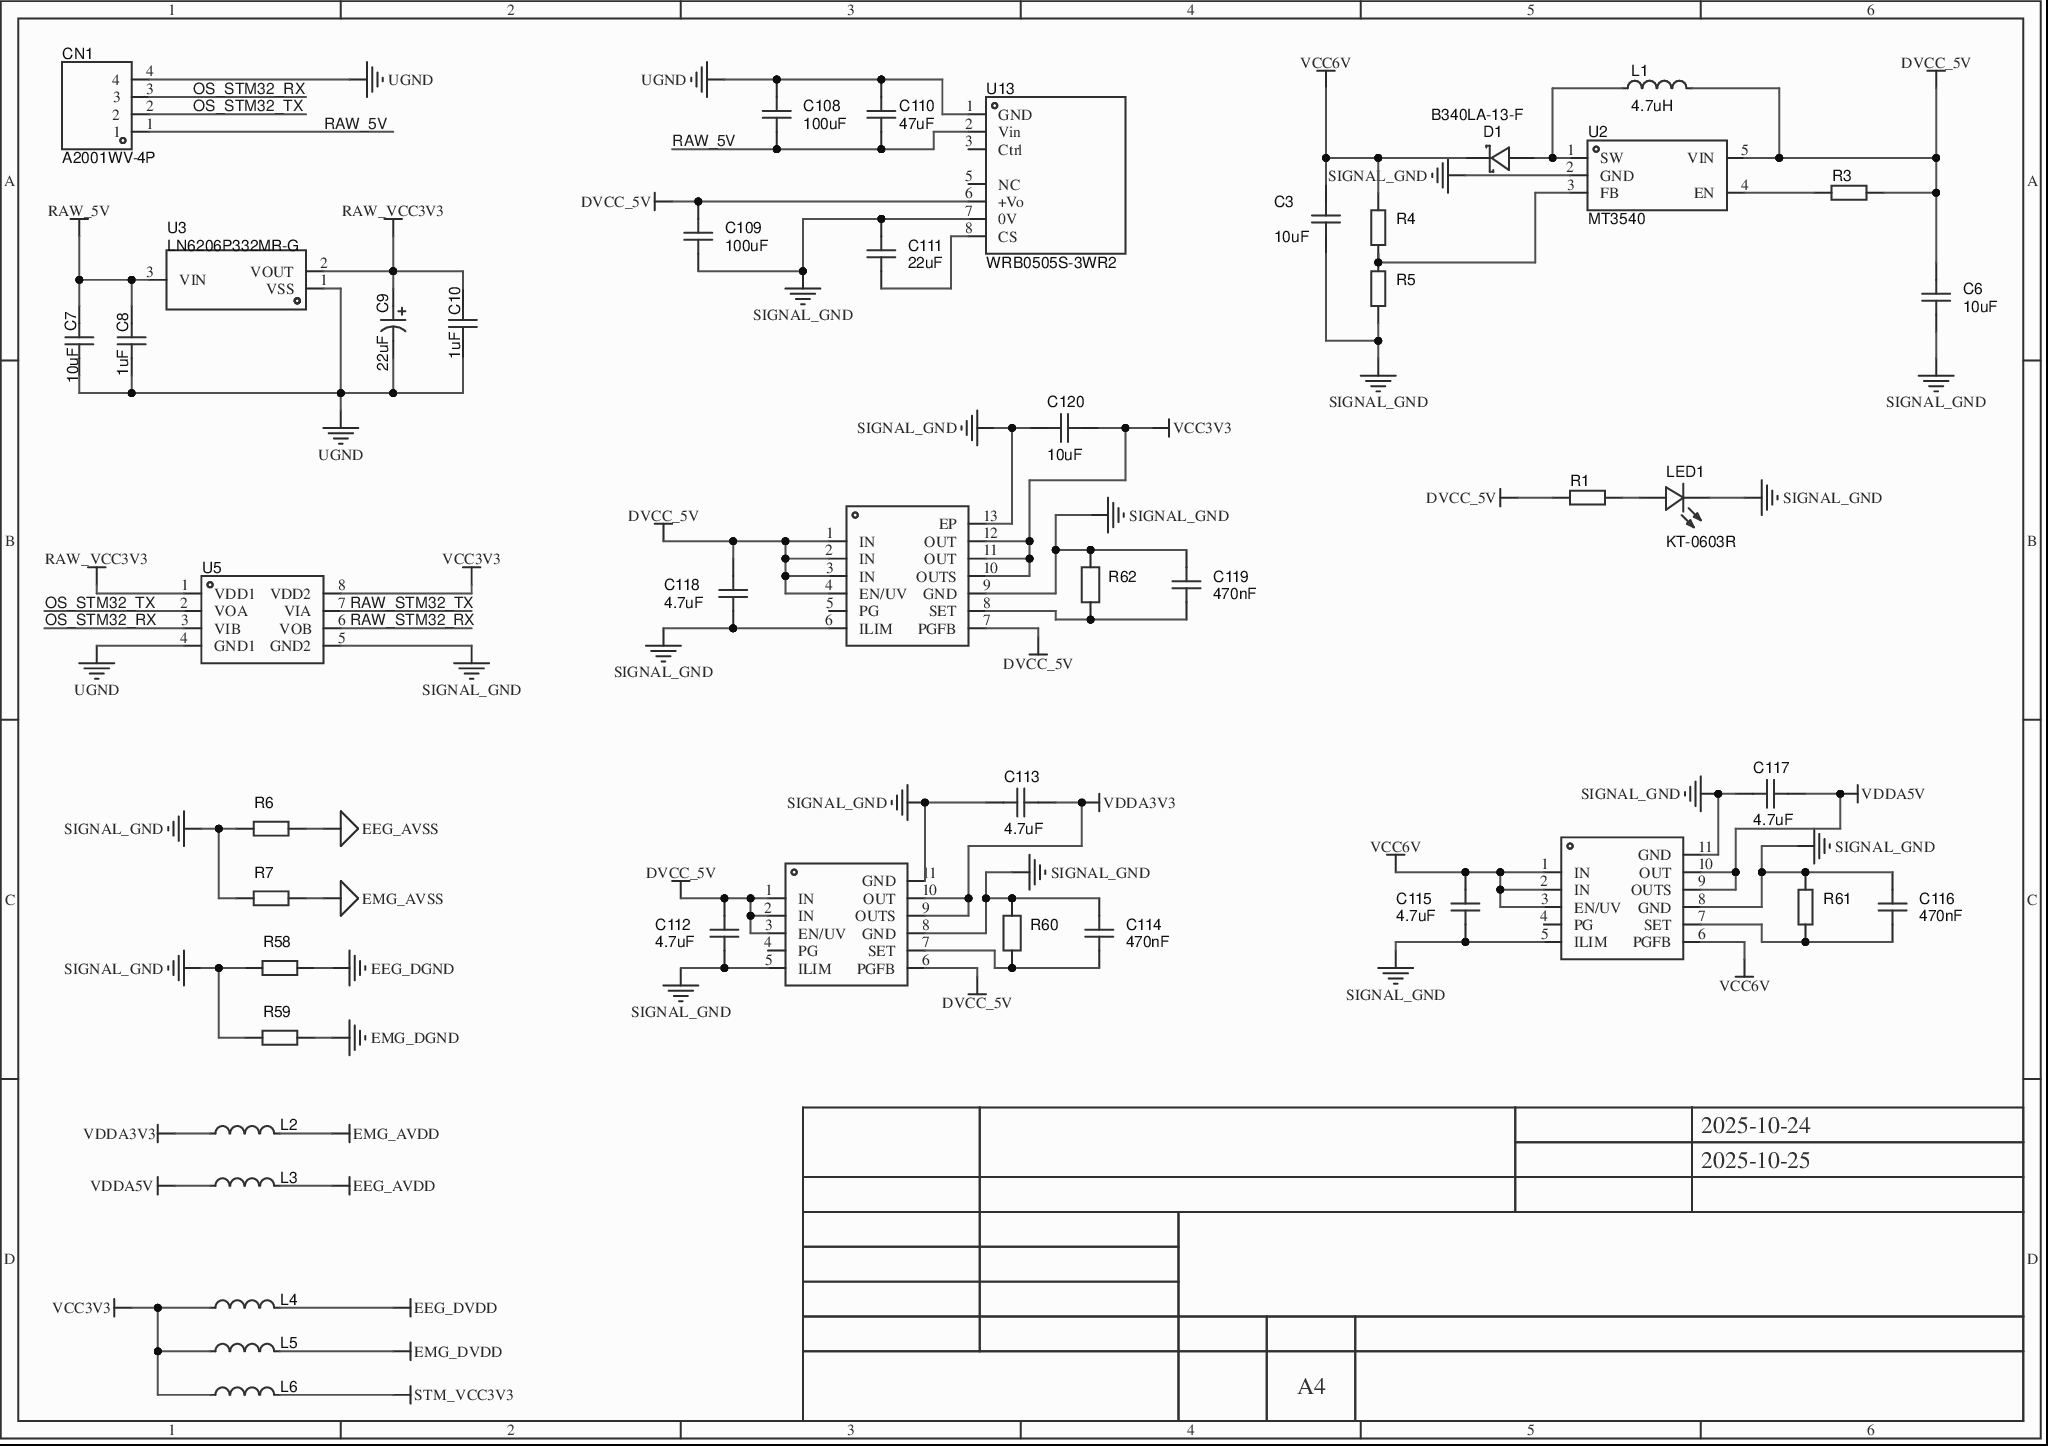
[diagram p0: MISC86293-47.schdoc]
# Altium project MISC86293-17.PrjPCB (part 1 of 3)
8 sheets, 211 parts. Net scope: global (net labels, ports and power ports of the same name join across sheets).
Board file: MISC86293.PcbDoc
Sheets:
  MISC86293-47.schdoc
  MISC86293-6.schdoc
  MISC86293-8.schdoc
  MISC86293-4.schdoc
  MISC86293-12.schdoc
  MISC86293-21.schdoc
  MISC86293-14.schdoc
  MISC86293-10.schdoc

## Sheet MISC86293-47.schdoc
size 297 x 209 mm; Version: V1.0; @Project Name: MISC86293; @Page Count: 8; @Update Date: 2025-10-25; @Create Date: 2025-10-24; @Schematic Name: MISC86293; @Page No: 1; @Create Time: 20:02:05; @Update Time: 11:40:48; @Board Name: MISC86293

### Parts
C3  10uF  [C0603]
C6  10uF  [C0603]
C7  10uF  [C0603]
C8  1uF  [C0402]
C9  22uF  [CAP-SMD_L3.2-W1.6]
C10  1uF  [C0402]
C108  100uF  [C1206]
C109  100uF  [C1206]
C110  47uF  [C1206]
C111  22uF  [C1206]
C112  4.7uF  [C0603]
C113  4.7uF  [C0603]
C114  470nF  [C0603]
C115  4.7uF  [C0603]
C116  470nF  [C0603]
C117  4.7uF  [C0603]
C118  4.7uF  [C0603]
C119  470nF  [C0603]
C120  10uF  [C0603]
CN1  A2001WV-4P  [CONN-TH_A2001WV-4P]
D1  B340LA-13-F  [SMA_L4.3-W2.6-LS5.2-RD]
L1  4.7uH  [IND-SMD_L4.0-W4.0_FNR40XXS]
L2  BLM15PD121SN1D  [L0402]  (value not drawn)
L3  BLM15PD121SN1D  [L0402]  (value not drawn)
L4  BLM15PD121SN1D  [L0402]  (value not drawn)
L5  BLM15PD121SN1D  [L0402]  (value not drawn)
L6  BLM15PD121SN1D  [L0402]  (value not drawn)
LED1  KT-0603R  [LED0603-RD]
R1  (no value)  [R0603]
R3  (no value)  [R0402]
R4  (no value)  [R0402]
R5  (no value)  [R0402]
R6  (no value)  [R0402]
R7  (no value)  [R0402]
R58  (no value)  [R0402]
R59  (no value)  [R0402]
R60  (no value)  [R0603]
R61  (no value)  [R0603]
R62  (no value)  [R0603]
U2  MT3540  [SOT-23-5_L3.0-W1.7-P0.95-LS2.8-BR]
U3  LN6206P332MR-G  [SOT-23-3_L2.9-W1.3-P1.90-LS2.4-BR]
U5  (no value)  [SOIC-8_L4.9-W3.9-P1.27-LS6.0-BL]
U13  WRB0505S-3WR2  [PWRM-TH_WRA0512S-3WR2]
U14  LT3045EMSE#TRPBF  [MSOP-12_L4.0-W3.0-P0.65-LS4.9-BL-EP]  (value not drawn)
U15  LT3042EMSE#TRPBF  [MSOP-10_L3.0-W3.0-P0.50-LS5.0-BL-EP]  (value not drawn)
U16  LT3042EMSE#TRPBF  [MSOP-10_L3.0-W3.0-P0.50-LS5.0-BL-EP]  (value not drawn)

### Nets
DVCC_5V: C6.2 C109.1 C112.2 C118.2 L1.2 R1.1 R3.2 U2.5(VIN) U13.6(+Vo) U14.1(IN) U14.2(IN) U14.3(IN) U14.4(EN/UV) U14.7(PGFB) U15.1(IN) U15.2(IN) U15.3(EN/UV) U15.6(PGFB)
EEG_AVDD: L3.2  [project net EEG_AVDD1]
EEG_AVSS: R6.1  [project net EEG_AVSS1]
EEG_DGND: R58.1  [project net EEG_DGND_1]
EEG_DVDD: L4.2  [project net EEG_DVDD_1]
EMG_AVDD: L2.2  [project net EMG_AVDD1]
EMG_AVSS: R7.1  [project net EMG_AVSS1]
EMG_DGND: R59.1  [project net EMG_DGND_1]
EMG_DVDD: L5.2  [project net EMG_DVDD_1]
RAW_5V: C7.2 C8.2 C108.1 C110.1 CN1.1 U3.3(VIN) U13.2(Vin)
RAW_VCC3V3: C9.1 C10.2 U3.2(VOUT) U5.1(VDD1)
SIGNAL_GND: C3.1 C6.1 C109.2 C111.2 C112.1 C113.2 C114.1 C115.1 C116.1 C117.2 C118.1 C119.1 C120.1 LED1.1(K) R5.1 R6.2 R7.2 R58.2 R59.2 R60.1 R61.2 R62.1 U2.2(GND) U5.5(GND2) U13.7(0V) U14.6(ILIM) U14.9(GND) U14.13(EP) U15.5(ILIM) U15.8(GND) U15.11(GND) U16.5(ILIM) U16.8(GND) U16.11(GND)
STM_VCC3V3: L6.2
UGND: C7.1 C8.1 C9.2 C10.1 C108.2 C110.2 CN1.4 U3.1(VSS) U5.4(GND1) U13.1(GND)
VCC3V3: C120.2 L4.1 L5.1 L6.1 U5.8(VDD2) U14.10(OUTS) U14.11(OUT) U14.12(OUT)
VCC6V: C3.2 C115.2 D1.1(K) R4.2 U16.1(IN) U16.2(IN) U16.3(EN/UV) U16.6(PGFB)
VDDA3V3: C113.1 L2.1 U15.9(OUTS) U15.10(OUT)
VDDA5V: C117.1 L3.1 U16.9(OUTS) U16.10(OUT)
OS_STM32_RX: CN1.3 U5.3(VIB)
OS_STM32_TX: CN1.2 U5.2(VOA)
RAW_STM32_RX: U5.6(VOB)
RAW_STM32_TX: U5.7(VIA)
NetC111_1: C111.1 U13.8(CS)
NetC114_2: C114.2 R60.2 U15.7(SET)
NetC116_2: C116.2 R61.1 U16.7(SET)
NetC119_2: C119.2 R62.2 U14.8(SET)
NetD1_2: D1.2(A) L1.1 U2.1(SW)
NetLED1_2: LED1.2(A) R1.2
NetR3_1: R3.1 U2.4(EN)
NetR4_1: R4.1 R5.2 U2.3(FB)

Not connected (* = marked no-connect by the designer): U13 3(Ctrl)* 5(NC)*; U14 5(PG)*; U15 4(PG)*; U16 4(PG)*

### Notes on the sheet
- 1
- 2
- 3
- 4
- 5
- 6
- A
- B
- C
- 2025-10-24
- 2025-10-25
- D
- A4

### Library data of the parts
C3 C6 = CL10A106MA8NRNC: AddInBom: yes; ModelId: ac125912035d415993ca9572d50418b1; ModelName: C0603_L1.6-W0.8-H0.8; ModelTransform: 62.992,31.496,0,0,0,0,0,0,0; Voltage Rated: 25V; Temperature Coefficient: X5R; Symbol: CL10A106MA8NRNC; Device: CL10A106MA8NRNC; Supplier: LCSC; Manufacturer Part: CL10A106MA8NRNC; Value: 10uF; Supplier Part: C96446; Supplier Footprint: 0603; Datasheet: https://atta.szlcsc.com/upload/public/pdf/source/20160218/1457707763339.pdf; ConvertToPcb: yes; FootprintName: C0603
C7 = CL10A106KP8NNNC: AddInBom: yes; ModelId: ac125912035d415993ca9572d50418b1; ModelName: C0603_L1.6-W0.8-H0.8; ModelTransform: 62.992,31.496,0,0,0,0,0,0,0; Voltage Rated: 10V; Temperature Coefficient: X5R; Symbol: CL10A106KP8NNNC; Device: CL10A106KP8NNNC; Supplier: LCSC; Manufacturer Part: CL10A106KP8NNNC; Value: 10uF; Supplier Part: C19702; Supplier Footprint: 0603; Datasheet: https://atta.szlcsc.com/upload/public/pdf/source/20160218/1457707763339.pdf; ConvertToPcb: yes; FootprintName: C0603
C8 C10 = CL05A105KA5NQNC: AddInBom: yes; ModelId: 36a51122f27c49738f86b3bfa98863e0; ModelName: C0402_L1.0-W0.5-H0.5; ModelTransform: 39.37,19.685,0,0,0,0,0,0,0; Voltage Rated: 25V; Temperature Coefficient: X5R; Symbol: CL05A105KA5NQNC; Device: CL05A105KA5NQNC; SupplierPart: C52923; ManufacturerPart: CL05A105KA5NQNC; Supplier Footprint: 0402; JLCPCB Part Class: Basic Part; Datasheet: https://atta.szlcsc.com/upload/public/pdf/source/20160218/1457707763339.pdf; Supplier: LCSC; ConvertToPcb: yes; FootprintName: C0402; Value: 1uF
C9 = CA45-A-16V-22uF-K: AddInBom: yes; ModelId: 16e6b9a38ba84019a70b57c5f1368526; ModelTransform: 125.984,62.992,0,0,0,0,0,0,0; Rated Voltage: 16V; Device: CA45-A-16V-22uF-K; Symbol: CA45-A-16V-22UF-K; SupplierPart: C782264; ManufacturerPart: CA45-A-16V-22uF-K; Supplier Footprint: CASE-A-3216; Datasheet: https://atta.szlcsc.com/upload/public/pdf/source/20200909/C782264_D6D9C4EF3B25E81633C26A9294FBB820.pdf; Supplier: LCSC; ConvertToPcb: yes; FootprintName: CAP-SMD_L3.2-W1.6; ModelName: CAP-SMD_L3.2-W1.6; Value: 22uF
C108 C109 = GRM31CR61A107MEA8L: AddInBom: yes; ModelId: e4be705b945545a48e666415e3682bd8; ModelName: C1206_L3.2-W1.6-H1.3; ModelTransform: 125.984,62.992,0,0,0,0,0,0,0; Voltage Rating: 10V; Temperature Coefficient: X5R; Symbol: GRM31CR61A107MEA8L; Device: GRM31CR61A107MEA8L; Value: 100uF; SupplierPart: C883598; ManufacturerPart: GRM31CR61A107MEA8L; Supplier Footprint: 1206; JLCPCB Part Class: Extended Part; Datasheet: https://item.szlcsc.com/datasheet/GRM31CR61A107MEA8L/948963.html; Supplier: LCSC; ConvertToPcb: yes; FootprintName: C1206
C110 = GRM31CR61A476ME15L: AddInBom: yes; ModelId: e4be705b945545a48e666415e3682bd8; ModelName: C1206_L3.2-W1.6-H1.3; ModelTransform: 125.984,62.992,0,0,0,0,0,0,0; Voltage Rating: 10V; Temperature Coefficient: X5R; Symbol: GRM31CR61A476ME15L; Device: GRM31CR61A476ME15L; Value: 47uF; SupplierPart: C94034; ManufacturerPart: GRM31CR61A476ME15L; Supplier Footprint: 1206; JLCPCB Part Class: Extended Part; Datasheet: https://item.szlcsc.com/datasheet/GRM31CR61A476ME15L/95232.html; Supplier: LCSC; ConvertToPcb: yes; FootprintName: C1206
C111 = GRM31CR71A226KE15L: AddInBom: yes; ModelId: e4be705b945545a48e666415e3682bd8; ModelName: C1206_L3.2-W1.6-H1.3; ModelTransform: 125.984,62.992,0,0,0,0,0,0,0; Voltage Rating: 10V; Temperature Coefficient: X7R; Symbol: GRM31CR71A226KE15L; Device: GRM31CR71A226KE15L; Value: 22uF; SupplierPart: C91604; ManufacturerPart: GRM31CR71A226KE15L; Supplier Footprint: 1206; JLCPCB Part Class: Extended Part; Datasheet: https://item.szlcsc.com/datasheet/GRM31CR71A226KE15L/92793.html; Supplier: LCSC; ConvertToPcb: yes; FootprintName: C1206
C112 C113 C115 C117 C118 = GRM188Z71C475KE21D: AddInBom: yes; ModelId: ac125912035d415993ca9572d50418b1; ModelName: C0603_L1.6-W0.8-H0.8; ModelTransform: 62.992,31.496,0,0,0,0,0,0,0; Voltage Rating: 16V; Temperature Coefficient: X7R; Symbol: GRM188Z71C475KE21D; Device: GRM188Z71C475KE21D; Value: 4.7uF; SupplierPart: C389010; ManufacturerPart: GRM188Z71C475KE21D; Supplier Footprint: 0603; JLCPCB Part Class: Extended Part; Datasheet: https://item.szlcsc.com/datasheet/GRM188Z71C475KE21D/364359.html; Supplier: LCSC; ConvertToPcb: yes; FootprintName: C0603
C114 C116 C119 = GRM188R71A474KA61D: AddInBom: yes; ModelId: ac125912035d415993ca9572d50418b1; ModelName: C0603_L1.6-W0.8-H0.8; ModelTransform: 62.992,31.496,0,0,0,0,0,0,0; Voltage Rating: 10V; Temperature Coefficient: X7R; Symbol: GRM188R71A474KA61D; Device: GRM188R71A474KA61D; Value: 470nF; SupplierPart: C435402; ManufacturerPart: GRM188R71A474KA61D; Supplier Footprint: 0603; JLCPCB Part Class: Extended Part; Datasheet: https://item.szlcsc.com/datasheet/GRM188R71A474KA61D/432740.html; Supplier: LCSC; ConvertToPcb: yes; FootprintName: C0603
C120 = GRM188Z71A106KA73D: AddInBom: yes; ModelId: ac125912035d415993ca9572d50418b1; ModelName: C0603_L1.6-W0.8-H0.8; ModelTransform: 62.992,31.496,0,0,0,0,0,0,0; Voltage Rated: 10V; Temperature Coefficient: X7R; Symbol: GRM188Z71A106KA73D; Device: GRM188Z71A106KA73D; SupplierPart: C2959727; ManufacturerPart: GRM188Z71A106KA73D; Supplier Footprint: 0603; JLCPCB Part Class: Extended Part; Datasheet: https://atta.szlcsc.com/upload/public/pdf/source/20220328/6A4892B7E841253269A84FFE395E0578.pdf; Supplier: LCSC; ConvertToPcb: yes; FootprintName: C0603; Value: 10uF
CN1 = A2001WV-4P: AddInBom: yes; ModelId: ab03000c925549fab984f1c356d5a65e; ModelName: PH2.0-LI-4P; ModelTransform: 393.701,186.908,0,180,0,0,0,19.685,-118.11; Pins Structure: 1x4P; Pitch: 2mm; Reference Series: PH; Number of PINs Per Row: 4; Current Rating: 2A; Voltage Rating: 100V; Plastic Material: PA66; Flame Retardant Rating: UL94V-0; Symbol: A2001WV-4P; Device: A2001WV-4P; SupplierPart: C225190; ManufacturerPart: A2001WV-4P; Datasheet: https://item.szlcsc.com/datasheet/A2001WV-4P/225473.html; Supplier: LCSC; ConvertToPcb: yes; FootprintName: CONN-TH_A2001WV-4P; Number of Pins: 4P; Number of Rows: 1; Row Spacing: -; Color: -
D1 = B340LA-13-F: AddInBom: yes; ModelId: 7ed2c9d0a4a74bbdbba07ab4052caf5b; ModelTransform: 185.039,102.362,0,0,0,0,0,0,0; Forward Voltage (Vf@If): 450mV@3A; Reverse Voltage (Vr): 40V; Average Rectified Current (Io): 3A; Reverse Leakage Current (Ir): 2mA@40V; Symbol: B340LA-13-F; Device: B340LA-13-F; Supplier: LCSC; Manufacturer Part: B340LA-13-F; Supplier Part: C17101; Supplier Footprint: SMA(DO-214AC); Datasheet: https://atta.szlcsc.com/upload/public/pdf/source/20171023/C97318_15087455366241052881.pdf; ConvertToPcb: yes; FootprintName: SMA_L4.3-W2.6-LS5.2-RD; ModelName: SMA_L4.3-W2.6-LS5.2-RD
L1 = FNR4030S4R7MT: AddInBom: yes; ModelId: f10f9856fbf34a8a9250995f07743de3; ModelName: IND-SMD_L4.0-W4.0-H2.6_FNR40XXS; ModelTransform: 157.48,157.48,0,270,0,0,0,0,0; Rated Current: 2.3A; Saturation Current (Isat): 3.2A; Symbol: FNR4030S4R7MT; Device: FNR4030S4R7MT; SupplierPart: C167874; ManufacturerPart: FNR4030S4R7MT; Supplier Footprint: SMD,4x4mm; Datasheet: https://atta.szlcsc.com/upload/public/pdf/source/20190327/C167925_9EFF0AABC4CA629C2CC95961DBF7D39D.pdf; Supplier: LCSC; ConvertToPcb: yes; FootprintName: IND-SMD_L4.0-W4.0_FNR40XXS; Value: 4.7uH
L2-L6 = BLM15PD121SN1D: AddInBom: yes; ModelId: d8d36575a3234d4790bfa765c88664a7; ModelName: L0402_L1.0-W0.5-H0.5_BEAD; ModelTransform: 39.37,19.685,0,0,0,0,0,0.0005,0; Current Rating: 1.3A; Circuits: 1; Device: BLM15PD121SN1D; Symbol: BLM15PD121SN1D; SupplierPart: C76891; ManufacturerPart: BLM15PD121SN1D; Supplier Footprint: 0402; Datasheet: https://atta.szlcsc.com/upload/public/pdf/source/20181120/C333978_3E581FB55966932B05020139ABDE8E01.pdf; Supplier: LCSC; ConvertToPcb: yes; FootprintName: L0402
LED1 = KT-0603R: Manufacturer: KENTO; AddInBom: yes; ModelId: 1f0d29a91be547639d425604e9b96ebb; ModelTransform: 63.7794,32.283,0,0,0,0,0,0,0; Symbol: KT-0603R; Device: KT-0603R; SupplierPart: C2286; ManufacturerPart: KT-0603R; Supplier Footprint: 0603; Datasheet: https://atta.szlcsc.com/upload/public/pdf/source/20160616/1466072038404.pdf; Supplier: LCSC; ConvertToPcb: yes; FootprintName: LED0603-RD; ModelName: LED0603-RD; Power Dissipation: -; Forward Current: -; Dominant Wavelength: -; Peak Wavelength: -; Diode Configuration: -; Lens Color: -; Color Temperature: -; Viewing Angle: -; Mounting Sytle: -
R1 = 0603WAF1001T5E: AddInBom: yes; ModelId: fc143cca1e79419f9cd78b61e9279f08; ModelTransform: 31.8897,63.7794,0,90,0,0,0,0,0; Power(Watts): 100mW; Overload Voltage (Max): 75V; Symbol: 0603WAF1001T5E; Device: 0603WAF1001T5E; SupplierPart: C21190; ManufacturerPart: 0603WAF1001T5E; Supplier Footprint: 0603; Datasheet: https://atta.szlcsc.com/upload/public/pdf/source/20200306/C422600_1E6D84923E4A46A82E41ADD87F860B5C.pdf; Supplier: LCSC; ConvertToPcb: yes; FootprintName: R0603; ModelName: R0603
R3 R5 = RC0402FR-0710KL: AddInBom: yes; ModelId: 671aefced39d4c318694bba8bd8efd39; ModelName: R0402_L1.0-W0.5-H0.5; ModelTransform: 39.37,19.685,0,0,0,0,0,0.0005,0; Power(Watts): 62.5mW; Overload Voltage (Max): 50V; Symbol: RC0402FR-0710KL; Device: RC0402FR-0710KL; SupplierPart: C60490; ManufacturerPart: RC0402FR-0710KL; Supplier Footprint: 0402; Datasheet: https://atta.szlcsc.com/upload/public/pdf/source/20170925/C131467_1506321478108990263.pdf; Supplier: LCSC; ConvertToPcb: yes; FootprintName: R0402
R4 = 0402WGF4022TCE: AddInBom: yes; ModelId: 671aefced39d4c318694bba8bd8efd39; ModelName: R0402_L1.0-W0.5-H0.5; ModelTransform: 39.37,19.685,0,0,0,0,0,0.0005,0; Power(Watts): 62.5mW; Overload Voltage (Max): 50V; Symbol: 0402WGF4022TCE; Device: 0402WGF4022TCE; Supplier: LCSC; Manufacturer Part: 0402WGF4022TCE; Supplier Part: C25893; Supplier Footprint: 0402; Datasheet: https://atta.szlcsc.com/upload/public/pdf/source/20200306/C422600_1E6D84923E4A46A82E41ADD87F860B5C.pdf; ConvertToPcb: yes; FootprintName: R0402
R6 R7 R58 R59 = 0402WGJ0000TCE: AddInBom: yes; ModelId: 671aefced39d4c318694bba8bd8efd39; ModelName: R0402_L1.0-W0.5-H0.5; ModelTransform: 39.37,19.685,0,0,0,0,0,0.0005,0; Power(Watts): 62.5mW; Overload Voltage (Max): 50V; Symbol: 0402WGJ0000TCE; Device: 0402WGJ0000TCE; SupplierPart: C21376; ManufacturerPart: 0402WGJ0000TCE; Supplier Footprint: 0402; JLCPCB Part Class: Extended Part; Datasheet: https://atta.szlcsc.com/upload/public/pdf/source/20200306/C422600_1E6D84923E4A46A82E41ADD87F860B5C.pdf; Supplier: LCSC; ConvertToPcb: yes; FootprintName: R0402
R60 R62 = 0603WAD3322T5E: AddInBom: yes; ModelId: fc143cca1e79419f9cd78b61e9279f08; ModelTransform: 31.8897,63.7794,0,90,0,0,0,0,0; Power(Watts): 100mW; Overload Voltage (Max): 75V; Symbol: 0603WAD3322T5E; Device: 0603WAD3322T5E; SupplierPart: C423044; ManufacturerPart: 0603WAD3322T5E; Supplier Footprint: 0603; JLCPCB Part Class: Extended Part; Datasheet: https://atta.szlcsc.com/upload/public/pdf/source/20200306/C422600_1E6D84923E4A46A82E41ADD87F860B5C.pdf; Supplier: LCSC; ConvertToPcb: yes; FootprintName: R0603; ModelName: R0603
R61 = 0603WAF4992T5E: AddInBom: yes; ModelId: fc143cca1e79419f9cd78b61e9279f08; ModelTransform: 31.8897,63.7794,0,90,0,0,0,0,0; Power(Watts): 100mW; Voltage-Supply(Max): 75V; Symbol: 0603WAF4992T5E; Device: 0603WAF4992T5E; SupplierPart: C23184; ManufacturerPart: 0603WAF4992T5E; Supplier Footprint: 0603; JLCPCB Part Class: Basic Part; Datasheet: https://item.szlcsc.com/datasheet/0603WAF4992T5E/23911.html; Supplier: LCSC; ConvertToPcb: yes; FootprintName: R0603; ModelName: R0603
U2 = MT3540: AddInBom: yes; ModelId: 0a2a1b8f50944f73965918ad6e5fe167; ModelName: SOT-23-5_L2.9-W1.6-H1.1-LS2.8-P0.95; ModelTransform: 114.173,109.636,0,180,0,0,0,0,0; Input Voltage: 2.5V~5.5V; Output Voltage: 28V; Output Current (Max): 1.5A; Switching Frequency: 1.2MHz; Number of Outputs: 1; Device: MT3540; Symbol: MT3540; LCSC Part Name: MT3540; SupplierPart: C181744; ManufacturerPart: MT3540; Supplier Footprint: SOT-23-5; Datasheet: https://atta.szlcsc.com/upload/public/pdf/source/20220425/7A219F2F25275A8C2665681DD7C42929.pdf; Supplier: LCSC; ConvertToPcb: yes; FootprintName: SOT-23-5_L3.0-W1.7-P0.95-LS2.8-BR; Synchronous Rectification: -
U3 = LN6206P332MR-G: AddInBom: yes; ModelId: c62791f0466c4ae2a892c056b845b0ca; ModelName: SOT-23-3P_L2.9-W1.3-H1.0-LS2.4-P0.95; ModelTransform: 98.425,114.173,0,180,0,0,0.0005,-0.0005,0; Maximum Input Voltage: 6V; Output Voltage: 3.3V; MAX Output Current: 250mA; Power Supply Rejection Ratio (PSRR): 40dB@(1kHz); Dropout Voltage: 240mV@(50mA); Number of Outputs: 1; Device: LN6206P332MR-G; Symbol: LN6206P332MR-G; SupplierPart: C141407; ManufacturerPart: LN6206P332MR-G; Supplier Footprint: SOT-23-3L; JLCPCB Part Class: Extended Part; Datasheet: https://atta.szlcsc.com/upload/public/pdf/source/20171110/C141415_15102792333721104208.pdf; Supplier: LCSC; ConvertToPcb: yes; FootprintName: SOT-23-3_L2.9-W1.3-P1.90-LS2.4-BR
U5 = _122M31: AddInBom: yes; ModelId: e81d2f7d937b4a6ab1dca543ff5d56a4; ModelName: SOIC-8_L4.9-W3.9-H1.7-LS6.0-P1.27; ModelTransform: 189.751,236.22,0,0,0,0,0.0005,0.0005,0; Number of Forward Channels: 1; Data Rate(Max): 10Mbps; Isolation Voltage(Vrms): 3000; CMTI(kV/us): 75kV/us; SupplierPart: C471594; Supplier Footprint: SOIC-8; Datasheet: https://item.szlcsc.com/datasheet/%25CF%2580122M31/478036.html; Supplier: LCSC; ConvertToPcb: yes; FootprintName: SOIC-8_L4.9-W3.9-P1.27-LS6.0-BL; Number of Reverse Channels: 1; Default Output: -
U13 = WRB0505S-3WR2: AddInBom: yes; ModelId: 8cc56816445444389b33bc96b9d6cdd4; ModelTransform: 866.14,374.802,0,0,0,0,0,-88.583,-161.417; Number of Channels: 1; Output Power: 3W; Voltage - Supply: 4.5V~9V; Conversion Efficiency: 73%; Output Voltage: 5V; Output Current(Max): 500mA; Isolation Voltage(Vrms): 1.5kV; Symbol: WRB0505S-3WR2; Device: WRB0505S-3WR2; Manufacturer Part: WRB0505S-3WR2; LCSC Part Name: WRB0505S-3WR2; SupplierPart: C44495; Supplier Footprint: SIP,22x9.5mm; JLCPCB Part Class: Extended Part; Datasheet: https://item.szlcsc.com/datasheet/WRB0505S-3WR2/45497.html; Supplier: LCSC; ConvertToPcb: yes; FootprintName: PWRM-TH_WRA0512S-3WR2; ModelName: PWRM-TH_WRA0512S-3WR2
U14 = LT3045EMSE#TRPBF: AddInBom: yes; ModelId: 67d385656a9548c0874f92c63457c823; ModelName: MSOP-12_L4.0-W3.0-H1.1-P0.65-LS4.9-BL-EP; ModelTransform: 157.48,192.913,0,0,0,0,0,0,0; Voltage - Supply: 20V; Output Voltage: 0V~15V; Output Current: 500mA; Power Supply Rejection Ratio (PSRR): 76dB@(1MHz); Voltage Dropout: 260mV@(500mA); Noise: 0.8uVrms; Number of Outputs: 1; Symbol: LT3045EMSE#TRPBF; Device: LT3045EMSE#TRPBF; SupplierPart: C666577; ManufacturerPart: LT3045EMSE#TRPBF; Supplier Footprint: MSOP-12-EP; JLCPCB Part Class: Extended Part; Datasheet: https://item.szlcsc.com/datasheet/LT3045EMSE%2523TRPBF/695863.html; Supplier: LCSC; ConvertToPcb: yes; FootprintName: MSOP-12_L4.0-W3.0-P0.65-LS4.9-BL-EP
U15 U16 = LT3042EMSE#TRPBF: AddInBom: yes; ModelId: 24a4fab644ec4e119b03a4a743393905; ModelName: MSOP-10_L3.0-W3.0-H1.1-LS5.0-P0.50; ModelTransform: 118.11,196.85,0,0,0,0,0,0,0; Maximum Input Voltage: 20V; Output Voltage: 0V~15V; Output Current: 200mA; Dropout Voltage: 350mV@(200mA); Number of Outputs: 1; Symbol: LT3042EMSE#TRPBF; Device: LT3042EMSE#TRPBF; SupplierPart: C461518; ManufacturerPart: LT3042EMSE#TRPBF; Supplier Footprint: MSOP-10-EP; JLCPCB Part Class: Extended Part; Datasheet: https://atta.szlcsc.com/upload/public/pdf/source/20191125/C461518_D70E324BD4D3ECAF70A76CB5055CFBFB.pdf; Supplier: LCSC; ConvertToPcb: yes; FootprintName: MSOP-10_L3.0-W3.0-P0.50-LS5.0-BL-EP; standby current: -; Noise: -

## Sheet MISC86293-6.schdoc
size 297 x 209 mm; Version: V1.0; @Project Name: MISC86293; @Page Count: 8; @Update Date: 2025-10-25; @Create Date: 2025-10-24; @Schematic Name: MISC86293; @Page No: 4; @Create Time: 20:02:05; @Update Time: 00:34:44; @Board Name: MISC86293
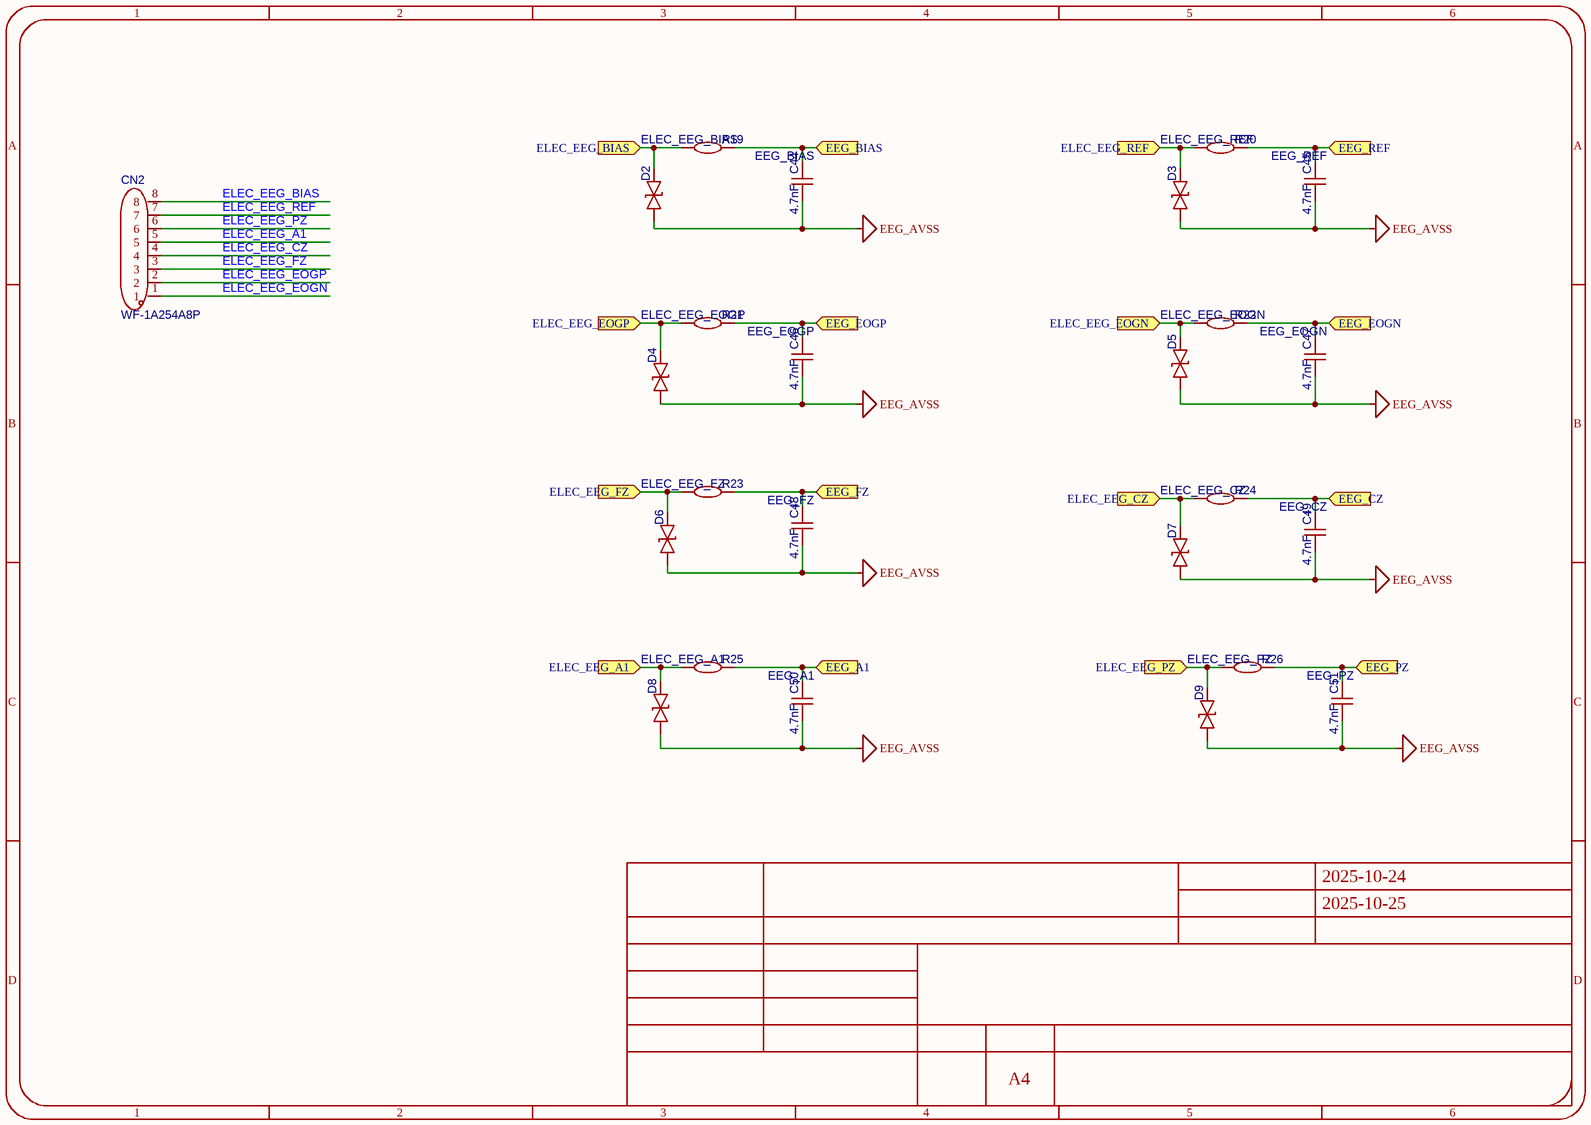
[diagram p1: MISC86293-6.schdoc]

### Parts
C44  4.7nF  [C0402]
C45  4.7nF  [C0402]
C46  4.7nF  [C0402]
C47  4.7nF  [C0402]
C48  4.7nF  [C0402]
C49  4.7nF  [C0402]
C50  4.7nF  [C0402]
C51  4.7nF  [C0402]
CN2  WF-1A254A8P  [CONN-TH_WF-1A254A8P]
D2  TPD1E10B06DPYR-TP  [X1-DFN1006-2_L1.0-W0.6-BI]  (value not drawn)
D3  TPD1E10B06DPYR-TP  [X1-DFN1006-2_L1.0-W0.6-BI]  (value not drawn)
D4  TPD1E10B06DPYR-TP  [X1-DFN1006-2_L1.0-W0.6-BI]  (value not drawn)
D5  TPD1E10B06DPYR-TP  [X1-DFN1006-2_L1.0-W0.6-BI]  (value not drawn)
D6  TPD1E10B06DPYR-TP  [X1-DFN1006-2_L1.0-W0.6-BI]  (value not drawn)
D7  TPD1E10B06DPYR-TP  [X1-DFN1006-2_L1.0-W0.6-BI]  (value not drawn)
D8  TPD1E10B06DPYR-TP  [X1-DFN1006-2_L1.0-W0.6-BI]  (value not drawn)
D9  TPD1E10B06DPYR-TP  [X1-DFN1006-2_L1.0-W0.6-BI]  (value not drawn)
R19  (no value)  [R0402]
R20  (no value)  [R0402]
R21  (no value)  [R0402]
R22  (no value)  [R0402]
R23  (no value)  [R0402]
R24  (no value)  [R0402]
R25  (no value)  [R0402]
R26  (no value)  [R0402]

### Ports
EEG_A1 (in), EEG_BIAS (in), EEG_CZ (in), EEG_EOGN (in), EEG_EOGP (in), EEG_FZ (in), EEG_PZ (in), EEG_REF (in), ELEC_EEG_A1 (in), ELEC_EEG_BIAS (in), ELEC_EEG_CZ (in), ELEC_EEG_EOGN (in), ELEC_EEG_EOGP (in), ELEC_EEG_FZ (in), ELEC_EEG_PZ (in), ELEC_EEG_REF (in)

### Nets
EEG_AVSS: C44.1 C45.1 C46.1 C47.1 C48.1 C49.1 C50.1 C51.1 D2.1 D3.1 D4.1 D5.1 D6.1 D7.1 D8.1 D9.1  [project net EEG_AVSS1]
EEG_A1: C50.2 R25.2 ; port EEG_A1
EEG_BIAS: C44.2 R19.2 ; port EEG_BIAS
EEG_CZ: C49.2 R24.2 ; port EEG_CZ
EEG_EOGN: C47.2 R22.2 ; port EEG_EOGN
EEG_EOGP: C46.2 R21.2 ; port EEG_EOGP
EEG_FZ: C48.2 R23.2 ; port EEG_FZ
EEG_PZ: C51.2 R26.2 ; port EEG_PZ
EEG_REF: C45.2 R20.2 ; port EEG_REF
ELEC_EEG_A1: CN2.5 D8.2 R25.1 ; port ELEC_EEG_A1
ELEC_EEG_BIAS: CN2.8 D2.2 R19.1 ; port ELEC_EEG_BIAS
ELEC_EEG_CZ: CN2.4 D7.2 R24.1 ; port ELEC_EEG_CZ
ELEC_EEG_EOGN: CN2.1 D5.2 R22.1 ; port ELEC_EEG_EOGN
ELEC_EEG_EOGP: CN2.2 D4.2 R21.1 ; port ELEC_EEG_EOGP
ELEC_EEG_FZ: CN2.3 D6.2 R23.1 ; port ELEC_EEG_FZ
ELEC_EEG_PZ: CN2.6 D9.2 R26.1 ; port ELEC_EEG_PZ
ELEC_EEG_REF: CN2.7 D3.2 R20.1 ; port ELEC_EEG_REF

### Notes on the sheet
- 1
- 2
- 3
- 4
- 5
- 6
- A
- B
- C
- 2025-10-24
- 2025-10-25
- D
- A4

### Library data of the parts
C44-C51 = 0402B472K500NT: AddInBom: yes; ModelId: 36a51122f27c49738f86b3bfa98863e0; ModelName: C0402_L1.0-W0.5-H0.5; ModelTransform: 39.37,19.685,0,0,0,0,0,0,0; Voltage Rated: 50V; Temperature Coefficient: X7R; Symbol: 0402B472K500NT; Device: 0402B472K500NT; SupplierPart: C1538; ManufacturerPart: 0402B472K500NT; Supplier Footprint: 0402; Datasheet: https://atta.szlcsc.com/upload/public/pdf/source/20200305/C486355_26A10D38EF8C2A5C37091D0039909270.pdf; Supplier: LCSC; ConvertToPcb: yes; FootprintName: C0402; Value: 4.7nF
CN2 = WF-1A254A8P: AddInBom: yes; ModelId: 3bf5a77c842d469b9fd6bb175a66ddf3; ModelTransform: 885.825,232.6767,0,0,0,0,0,24.016,-133.858; Pins Structure: 1x8P; Pitch: 2.5mm; Reference Series: XH; Number of PINs Per Row: 8; Current Rating: 3A; Symbol: WF-1A254A8P; Device: WF-1A254A8P; SupplierPart: C23396997; ManufacturerPart: WF-1A254A8P; Datasheet: https://item.szlcsc.com/datasheet/WF-1A254A8P/25127783.html; Supplier: LCSC; ConvertToPcb: yes; FootprintName: CONN-TH_WF-1A254A8P; ModelName: CONN-TH_WF-1A254A8P; Number of Pins: 8P; Number of Rows: 1
D2-D9 = TPD1E10B06DPYR-TP: AddInBom: yes; ModelId: be5a8b78c3cb4e51be1cd7cc83308da0; ModelName: X1-DFN1006-2_L1.0-W0.6-H0.5-BI; ModelTransform: 40.1574,24.4094,0,0,0,0,0,0,0; Symbol: TPD1E10B06DPYR-TP; Device: TPD1E10B06DPYR-TP; Supplier: LCSC; Supplier Part: C558445; Manufacturer Part: TPD1E10B06DPYR-TP; LCSC Part Name: TPD1E10B06DPYR-TP; Supplier Footprint: X1-DFN1006-2; Datasheet: https://atta.szlcsc.com/upload/public/pdf/source/20230621/7FCA3FDEAE9F1BA71F34C850D9682567.pdf; ConvertToPcb: yes; FootprintName: X1-DFN1006-2_L1.0-W0.6-BI
R19-R26 = 0402WGF4991TCE: AddInBom: yes; ModelId: 671aefced39d4c318694bba8bd8efd39; ModelName: R0402_L1.0-W0.5-H0.5; ModelTransform: 39.37,19.685,0,0,0,0,0,0.0005,0; Power(Watts): 62.5mW; Overload Voltage (Max): 50V; Symbol: 0402WGF4991TCE; Device: 0402WGF4991TCE; Supplier: LCSC; Manufacturer Part: 0402WGF4991TCE; Supplier Part: C25903; JLCPCB Part Class: Extended Part; Supplier Footprint: 0402; Datasheet: https://atta.szlcsc.com/upload/public/pdf/source/20200306/C422600_1E6D84923E4A46A82E41ADD87F860B5C.pdf; ConvertToPcb: yes; FootprintName: R0402

## Sheet MISC86293-8.schdoc
size 297 x 209 mm; Version: V1.0; @Project Name: MISC86293; @Page Count: 8; @Update Date: 2025-10-14; @Create Date: 2025-10-12; @Schematic Name: MISC86293; @Page No: 3; @Create Time: 22:49:01; @Update Time: 19:43:59; @Board Name: MISC86293
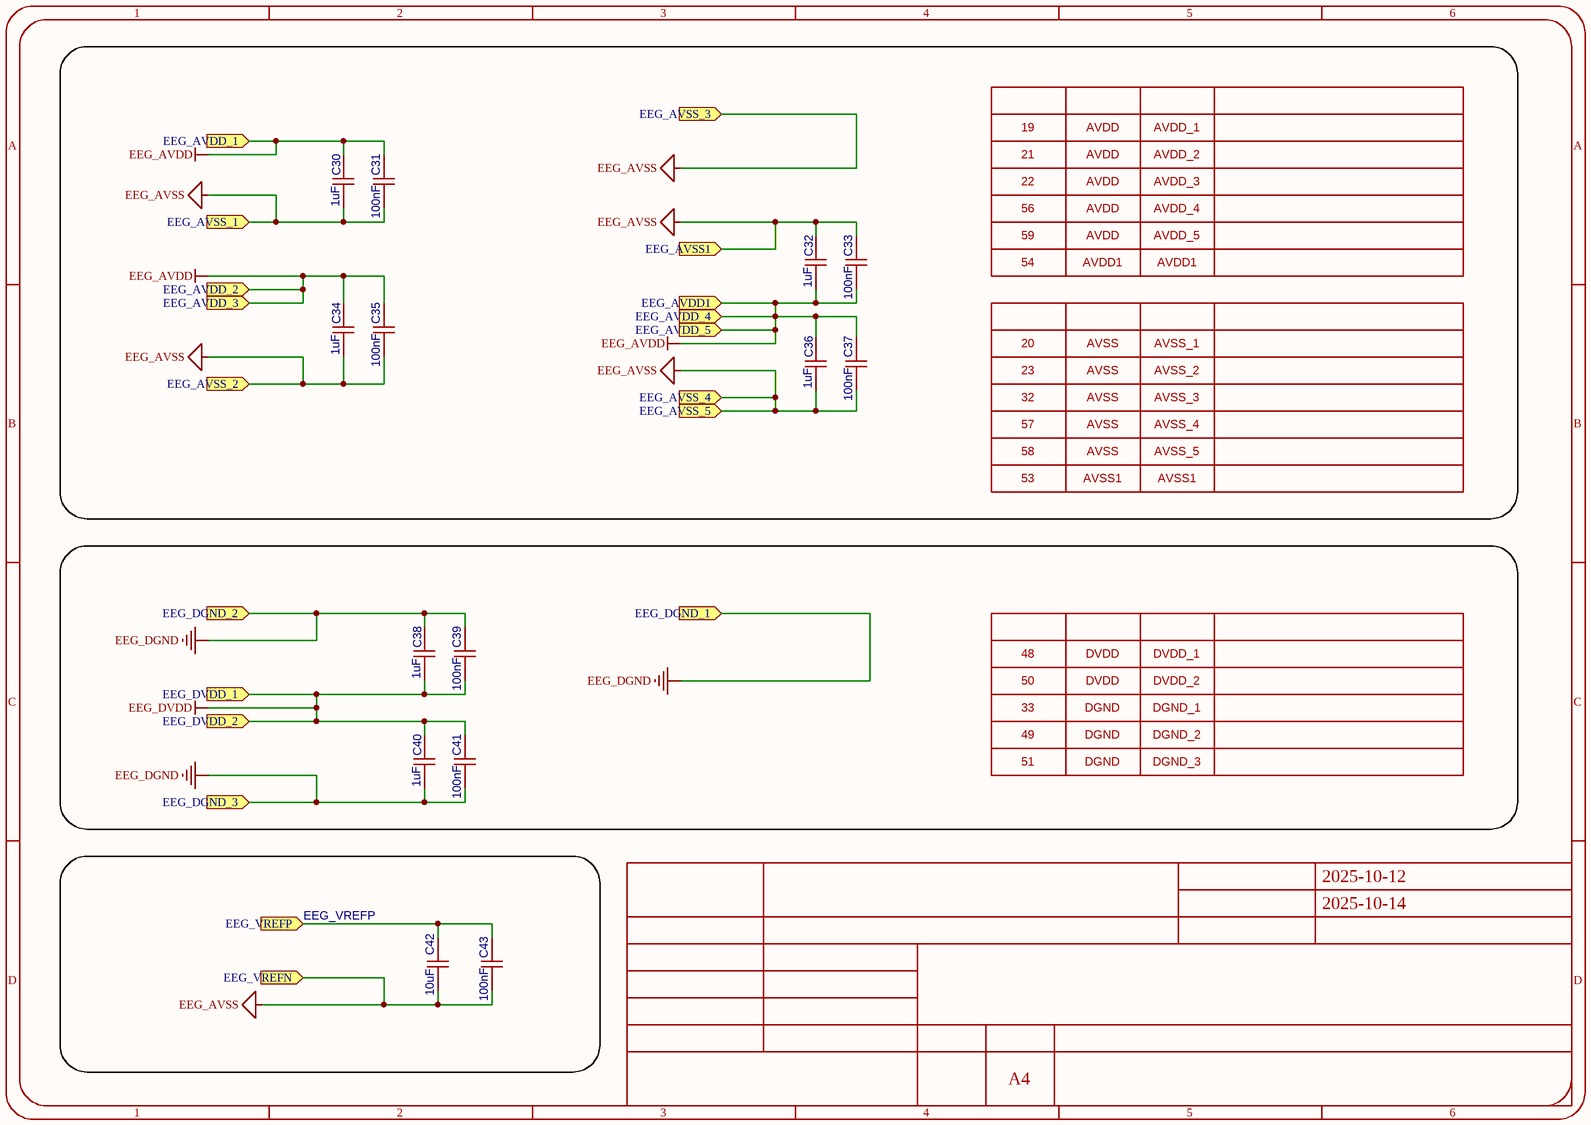
[diagram p2: MISC86293-8.schdoc]

### Parts
C30  1uF  [C0402]
C31  100nF  [C0402]
C32  1uF  [C0402]
C33  100nF  [C0402]
C34  1uF  [C0402]
C35  100nF  [C0402]
C36  1uF  [C0402]
C37  100nF  [C0402]
C38  1uF  [C0402]
C39  100nF  [C0402]
C40  1uF  [C0402]
C41  100nF  [C0402]
C42  10uF  [C0603]
C43  100nF  [C0402]

### Ports
EEG_AVDD1 (in), EEG_AVDD_1 (in), EEG_AVDD_2 (in), EEG_AVDD_3 (in), EEG_AVDD_4 (in), EEG_AVDD_5 (in), EEG_AVSS1 (in), EEG_AVSS_1 (in), EEG_AVSS_2 (in), EEG_AVSS_3 (in), EEG_AVSS_4 (in), EEG_AVSS_5 (in), EEG_DGND_1 (in), EEG_DGND_2 (in), EEG_DGND_3 (in), EEG_DVDD_1 (in), EEG_DVDD_2 (in), EEG_VREFN (in), EEG_VREFP (in)

### Nets
EEG_AVDD: C30.2 C31.2 C32.1 C33.1 C34.2 C35.2 C36.2 C37.2 ; port EEG_AVDD_1, port EEG_AVDD_2, port EEG_AVDD_3, port EEG_AVDD_4, port EEG_AVDD_5, port EEG_AVDD1  [project net EEG_AVDD1]
EEG_AVSS: C30.1 C31.1 C32.2 C33.2 C34.1 C35.1 C36.1 C37.1 C42.1 C43.1 ; port EEG_AVSS_1, port EEG_AVSS_2, port EEG_AVSS_3, port EEG_AVSS_4, port EEG_AVSS_5, port EEG_VREFN, port EEG_AVSS1  [project net EEG_AVSS1]
EEG_DGND: C38.2 C39.2 C40.1 C41.1 ; port EEG_DGND_1, port EEG_DGND_2, port EEG_DGND_3  [project net EEG_DGND_1]
EEG_DVDD: C38.1 C39.1 C40.2 C41.2 ; port EEG_DVDD_2, port EEG_DVDD_1  [project net EEG_DVDD_1]
EEG_VREFP: C42.2 C43.2 ; port EEG_VREFP

### Notes on the sheet
- 19
- AVDD
- AVDD_1
- 21
- 22
- 56
- AVDD_2
- AVDD_3
- AVDD_4
- 59
- 54
- AVDD1
- AVDD_5
- 20
- AVSS
- AVSS_1
- 23
- 32
- AVSS_2
- AVSS_3
- 57
- 58
- 53
- AVSS1
- AVSS_4
- AVSS_5
- 48
- 50
- DVDD
- DVDD_1
- DVDD_2
- 33
- 49
- DGND
- DGND_1
- DGND_2
- 51
- DGND_3
- 1
- 2
- 3
- 4
- 5
- 6
- A
- B
- C
- 2025-10-12
- 2025-10-14
- D
- A4

### Library data of the parts
C30 C32 C34 C36 C38 C40 = GRM155Z71A105KE01D: AddInBom: yes; ModelId: 36a51122f27c49738f86b3bfa98863e0; ModelName: C0402_L1.0-W0.5-H0.5; ModelTransform: 39.37,19.685,0,0,0,0,0,0,0; Voltage Rated: 10V; Temperature Coefficient: X7R; Symbol: GRM155Z71A105KE01D; Device: GRM155Z71A105KE01D; SupplierPart: C528974; ManufacturerPart: GRM155Z71A105KE01D; Supplier Footprint: 0402; Datasheet: https://atta.szlcsc.com/upload/public/pdf/source/20200508/C528974_15BC5D9F0CC13FAE313D74FE55DE6D9B.pdf; Supplier: LCSC; ConvertToPcb: yes; FootprintName: C0402; Value: 1uF
C31 C33 C35 C37 C39 C41 C43 = CL05B104KB54PNC: AddInBom: yes; ModelId: 36a51122f27c49738f86b3bfa98863e0; ModelName: C0402_L1.0-W0.5-H0.5; ModelTransform: 39.37,19.685,0,0,0,0,0,0,0; Voltage Rated: 50V; Temperature Coefficient: X7R; Device: CL05B104KB54PNC; Symbol: CL05B104KB54PNC; SupplierPart: C307331; ManufacturerPart: CL05B104KB54PNC; Supplier Footprint: 0402; Datasheet: https://atta.szlcsc.com/upload/public/pdf/source/20160218/1457707763339.pdf; Supplier: LCSC; ConvertToPcb: yes; FootprintName: C0402; Value: 100nF
C42 = CL10A106MA8NRNC: as C3 on sheet MISC86293-47; Symbol: CL10A106MA8NRNC; Device: CL10A106MA8NRNC; Supplier: LCSC; Manufacturer Part: CL10A106MA8NRNC; Value: 10uF; Supplier Part: C96446; Supplier Footprint: 0603; Datasheet: https://atta.szlcsc.com/upload/public/pdf/source/20160218/1457707763339.pdf; ConvertToPcb: yes; FootprintName: C0603